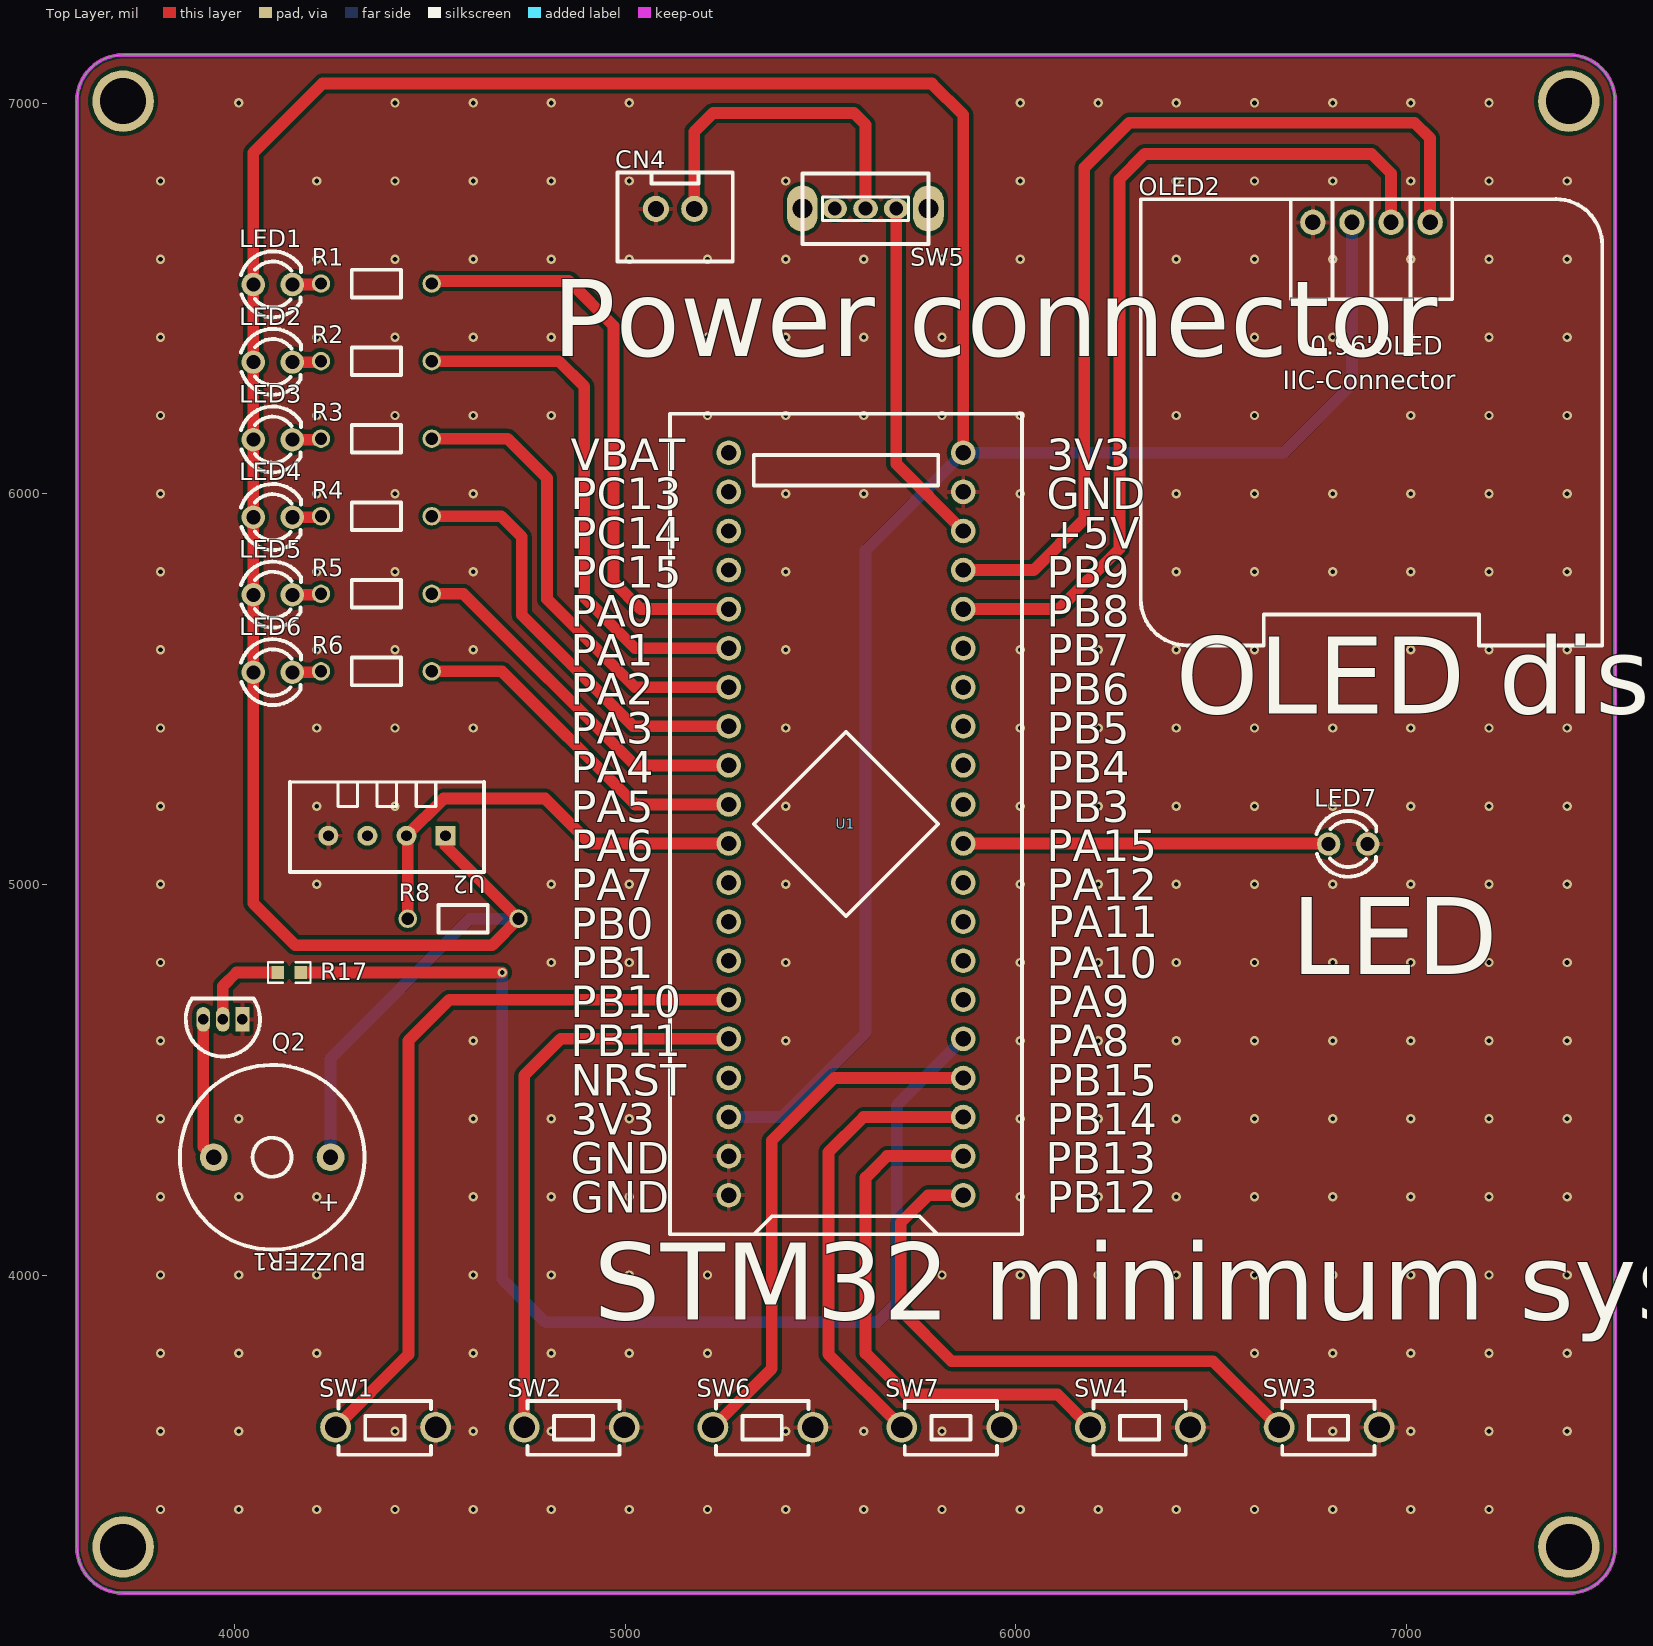
[diagram p0: Top Layer view]
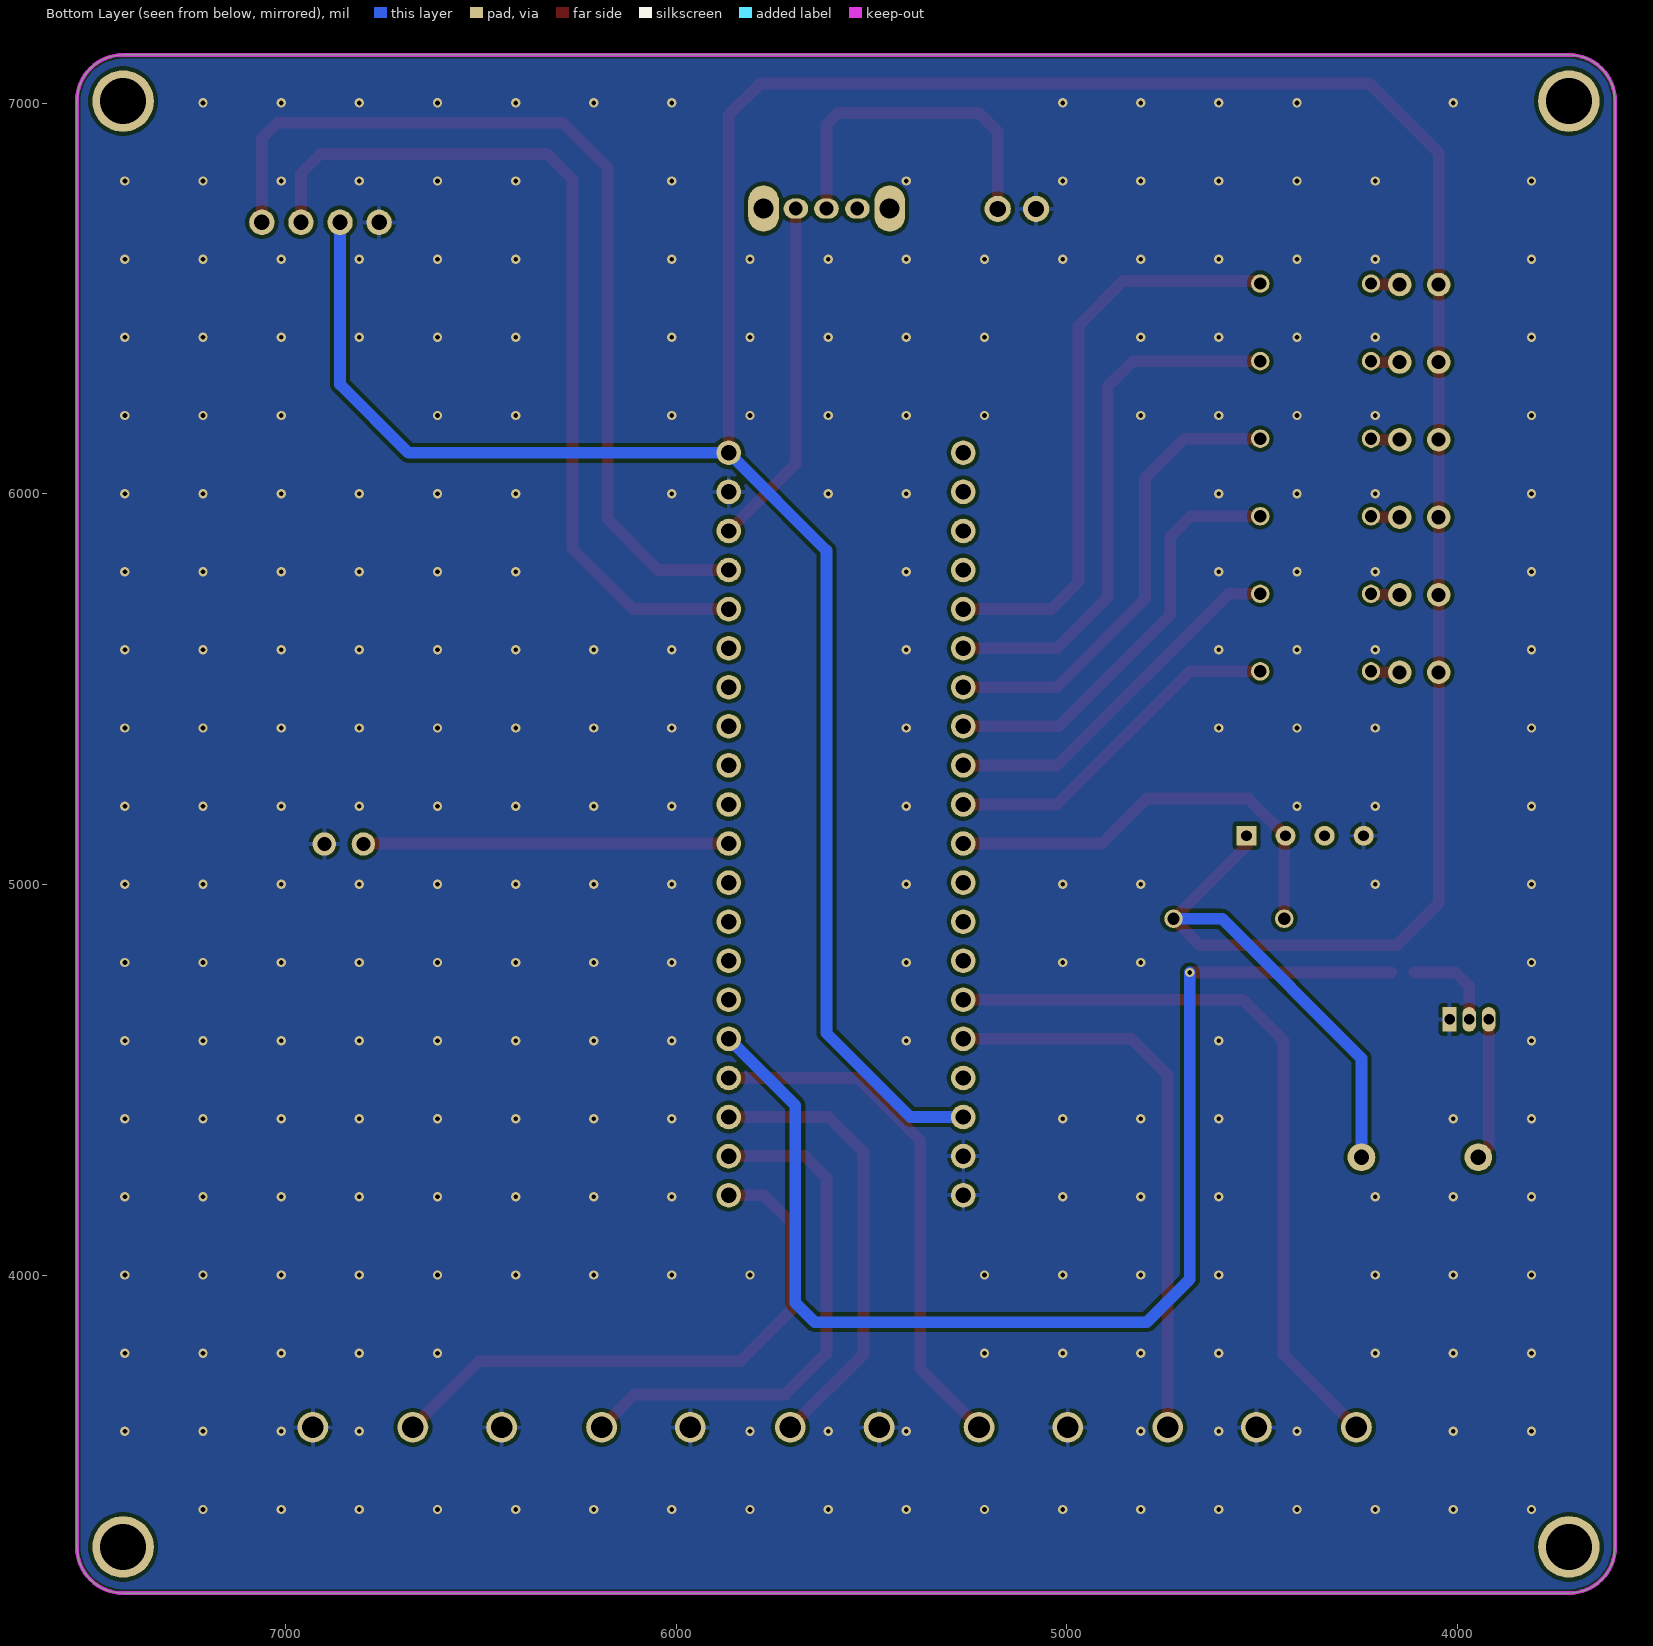
[diagram p1: Bottom Layer view, seen from below]
# Altium PCB MISC51258.pcbdoc
Units mil, origin at the board's own origin, x right, y up, seen from the top; angles counter-clockwise.
Board outline 3937.01 x 3937.01 mil, 2 copper layers (Top Layer, Bottom Layer), stack 62.206 mil thick; 28 components, 46 nets, 106 pads, 258 vias.

## Layer stack, top to bottom
Top Solder Mask Layer: solder mask 0.394, Dk 3.3
Top Layer: signal copper 1.379
Dielectric1: surface 59.449, FR4, Dk 4.5
Bottom Layer: signal copper 1.378
Bottom Solder Mask Layer: solder mask 0.394, Dk 3.3

## Board outline
3714.61,7123.5 ccw(c3714.61,7005.39) 3596.5,7005.39 3596.5,3304.61 ccw(c3714.61,3304.61) 3714.61,3186.5 7415.39,3186.5 ccw(c7415.39,3304.61) 7533.5,3304.61 7533.5,7005.39 ccw(c7415.39,7005.39) 7415.39,7123.5 3714.61,7123.5

## Design rules (kind name [scope] priority, off if disabled: settings)
BoardOutlineClearance copperThickness2oz_1 [All] p2 off: genericclearance=7.99 ignorepadtopadclearanceinfootprint=FALSE except(0: Arc-SplitContinuation Track-SplitContinuation SMDPad-SplitContinuation THPad-SplitContinuation Via-SplitContinuation Fill-SplitContinuation Region-SplitContinuation Poly-SplitContinuation Text-SplitContinuation Hole-SplitContinuation; 5.98: Arc-CutoutEdge Track-CutoutEdge SMDPad-CutoutEdge THPad-CutoutEdge Via-CutoutEdge Text-CutoutEdge; 6.9: Hole-OutlineEdge Hole-CutoutEdge; 10: Poly-OutlineEdge Poly-CutoutEdge; 11.81: Arc-OutlineEdge Track-OutlineEdge SMDPad-OutlineEdge THPad-OutlineEdge Via-OutlineEdge Fill-OutlineEdge Region-OutlineEdge Text-OutlineEdge Fill-CutoutEdge Region-CutoutEdge)
BoardOutlineClearance Plane_innerPlane_1 [All] p4 off: genericclearance=4.02 ignorepadtopadclearanceinfootprint=FALSE except(0: Arc-SplitContinuation Track-SplitContinuation SMDPad-SplitContinuation THPad-SplitContinuation Via-SplitContinuation Fill-SplitContinuation Region-SplitContinuation Poly-SplitContinuation Text-SplitContinuation Hole-SplitContinuation; 5.98: Arc-CutoutEdge Track-CutoutEdge SMDPad-CutoutEdge THPad-CutoutEdge Via-CutoutEdge Text-CutoutEdge; 6.9: Hole-OutlineEdge Hole-CutoutEdge; 10: Poly-OutlineEdge Poly-CutoutEdge; 11.81: Arc-OutlineEdge Track-OutlineEdge SMDPad-OutlineEdge THPad-OutlineEdge Via-OutlineEdge Fill-OutlineEdge Region-OutlineEdge Text-OutlineEdge Fill-CutoutEdge Region-CutoutEdge)
BoardOutlineClearance Copper_copperRegion_1 [All] p6 off: genericclearance=4.02 ignorepadtopadclearanceinfootprint=FALSE except(0: Arc-SplitContinuation Track-SplitContinuation SMDPad-SplitContinuation THPad-SplitContinuation Via-SplitContinuation Fill-SplitContinuation Region-SplitContinuation Poly-SplitContinuation Text-SplitContinuation Hole-SplitContinuation; 5.98: Arc-CutoutEdge Track-CutoutEdge SMDPad-CutoutEdge THPad-CutoutEdge Via-CutoutEdge Text-CutoutEdge; 6.9: Hole-OutlineEdge Hole-CutoutEdge; 10: Poly-OutlineEdge Poly-CutoutEdge; 11.81: Arc-OutlineEdge Track-OutlineEdge SMDPad-OutlineEdge THPad-OutlineEdge Via-OutlineEdge Fill-OutlineEdge Region-OutlineEdge Text-OutlineEdge Fill-CutoutEdge Region-CutoutEdge)
BoardOutlineClearance Copper_copperRegion_copperThickness1oz_1 [All] p8 off: genericclearance=4.02 ignorepadtopadclearanceinfootprint=FALSE except(0: Arc-SplitContinuation Track-SplitContinuation SMDPad-SplitContinuation THPad-SplitContinuation Via-SplitContinuation Fill-SplitContinuation Region-SplitContinuation Poly-SplitContinuation Text-SplitContinuation Hole-SplitContinuation; 5.98: Arc-CutoutEdge Track-CutoutEdge SMDPad-CutoutEdge THPad-CutoutEdge Via-CutoutEdge Text-CutoutEdge; 6.9: Hole-OutlineEdge Hole-CutoutEdge; 10: Poly-OutlineEdge Poly-CutoutEdge; 11.81: Arc-OutlineEdge Track-OutlineEdge SMDPad-OutlineEdge THPad-OutlineEdge Via-OutlineEdge Fill-OutlineEdge Region-OutlineEdge Text-OutlineEdge Fill-CutoutEdge Region-CutoutEdge)
BoardOutlineClearance Copper_copperRegion_Copper_copperRegion_1 [All] p10 off: genericclearance=4.02 ignorepadtopadclearanceinfootprint=FALSE except(0: Arc-SplitContinuation Track-SplitContinuation SMDPad-SplitContinuation THPad-SplitContinuation Via-SplitContinuation Fill-SplitContinuation Region-SplitContinuation Poly-SplitContinuation Text-SplitContinuation Hole-SplitContinuation; 5.98: Arc-CutoutEdge Track-CutoutEdge SMDPad-CutoutEdge THPad-CutoutEdge Via-CutoutEdge Text-CutoutEdge; 6.9: Hole-OutlineEdge Hole-CutoutEdge; 10: Poly-OutlineEdge Poly-CutoutEdge; 11.81: Arc-OutlineEdge Track-OutlineEdge SMDPad-OutlineEdge THPad-OutlineEdge Via-OutlineEdge Fill-OutlineEdge Region-OutlineEdge Text-OutlineEdge Fill-CutoutEdge Region-CutoutEdge)
BoardOutlineClearance copperThickness1oz_1 [All] p12: genericclearance=4.02 ignorepadtopadclearanceinfootprint=FALSE except(0: Arc-SplitContinuation Track-SplitContinuation SMDPad-SplitContinuation THPad-SplitContinuation Via-SplitContinuation Fill-SplitContinuation Region-SplitContinuation Poly-SplitContinuation Text-SplitContinuation Hole-SplitContinuation; 5.98: Arc-CutoutEdge Track-CutoutEdge SMDPad-CutoutEdge THPad-CutoutEdge Via-CutoutEdge Text-CutoutEdge; 6.9: Hole-OutlineEdge Hole-CutoutEdge; 10: Poly-OutlineEdge Poly-CutoutEdge; 11.81: Arc-OutlineEdge Track-OutlineEdge SMDPad-OutlineEdge THPad-OutlineEdge Via-OutlineEdge Fill-OutlineEdge Region-OutlineEdge Text-OutlineEdge Fill-CutoutEdge Region-CutoutEdge)
Clearance copperThickness2oz [All] p1 off: gap=7.99 ignorepadtopadclearanceinfootprint=FALSE except(5.98: SMDPad-Track SMDPad-SMDPad THPad-Track SMDPad-THPad THPad-THPad Track-Via SMDPad-Via THPad-Via Via-Via Fill-SMDPad Region-SMDPad Fill-THPad Region-THPad Fill-Via Region-Via Fill-Fill Fill-Region Region-Region Arc-Track Arc-SMDPad Arc-THPad Arc-Via Fill-Arc Region-Arc Arc-Arc Text-Track SMDPad-Text Text-THPad Text-Via Fill-Text Region-Text Arc-Text Text-Text; 6.9: Hole-Track Hole-SMDPad Hole-THPad Hole-Via Fill-Hole Region-Hole Hole-Arc Hole-Text; 10: Poly-Track Poly-SMDPad Poly-THPad Poly-Via Poly-Fill Poly-Region Poly-Poly Poly-Arc Poly-Text Poly-Hole; 11.81: Fill-Track Region-Track)
Clearance Plane_innerPlane [All] p3 off: gap=4.02 ignorepadtopadclearanceinfootprint=FALSE except(5.98: SMDPad-Track SMDPad-SMDPad THPad-Track SMDPad-THPad THPad-THPad Track-Via SMDPad-Via THPad-Via Via-Via Fill-SMDPad Region-SMDPad Fill-THPad Region-THPad Fill-Via Region-Via Fill-Fill Fill-Region Region-Region Arc-Track Arc-SMDPad Arc-THPad Arc-Via Fill-Arc Region-Arc Arc-Arc Text-Track SMDPad-Text Text-THPad Text-Via Fill-Text Region-Text Arc-Text Text-Text; 6.9: Hole-Track Hole-SMDPad Hole-THPad Hole-Via Fill-Hole Region-Hole Hole-Arc Hole-Text; 10: Poly-Track Poly-SMDPad Poly-THPad Poly-Via Poly-Fill Poly-Region Poly-Poly Poly-Arc Poly-Text Poly-Hole; 11.81: Fill-Track Region-Track)
Clearance Copper_copperRegion [All] p5 off: gap=4.02 ignorepadtopadclearanceinfootprint=FALSE except(5.98: SMDPad-Track SMDPad-SMDPad THPad-Track SMDPad-THPad THPad-THPad Track-Via SMDPad-Via THPad-Via Via-Via Fill-SMDPad Region-SMDPad Fill-THPad Region-THPad Fill-Via Region-Via Fill-Fill Fill-Region Region-Region Arc-Track Arc-SMDPad Arc-THPad Arc-Via Fill-Arc Region-Arc Arc-Arc Text-Track SMDPad-Text Text-THPad Text-Via Fill-Text Region-Text Arc-Text Text-Text; 6.9: Hole-Track Hole-SMDPad Hole-THPad Hole-Via Fill-Hole Region-Hole Hole-Arc Hole-Text; 10: Poly-Track Poly-SMDPad Poly-THPad Poly-Via Poly-Fill Poly-Region Poly-Poly Poly-Arc Poly-Text Poly-Hole; 11.81: Fill-Track Region-Track)
Clearance Copper_copperRegion_copperThickness1oz [All] p7 off: gap=4.02 ignorepadtopadclearanceinfootprint=FALSE except(5.98: SMDPad-Track SMDPad-SMDPad THPad-Track SMDPad-THPad THPad-THPad Track-Via SMDPad-Via THPad-Via Via-Via Fill-SMDPad Region-SMDPad Fill-THPad Region-THPad Fill-Via Region-Via Fill-Fill Fill-Region Region-Region Arc-Track Arc-SMDPad Arc-THPad Arc-Via Fill-Arc Region-Arc Arc-Arc Text-Track SMDPad-Text Text-THPad Text-Via Fill-Text Region-Text Arc-Text Text-Text; 6.9: Hole-Track Hole-SMDPad Hole-THPad Hole-Via Fill-Hole Region-Hole Hole-Arc Hole-Text; 10: Poly-Track Poly-SMDPad Poly-THPad Poly-Via Poly-Fill Poly-Region Poly-Poly Poly-Arc Poly-Text Poly-Hole; 11.81: Fill-Track Region-Track)
Clearance Copper_copperRegion_Copper_copperRegion [All] p9 off: gap=4.02 ignorepadtopadclearanceinfootprint=FALSE except(5.98: SMDPad-Track SMDPad-SMDPad THPad-Track SMDPad-THPad THPad-THPad Track-Via SMDPad-Via THPad-Via Via-Via Fill-SMDPad Region-SMDPad Fill-THPad Region-THPad Fill-Via Region-Via Fill-Fill Fill-Region Region-Region Arc-Track Arc-SMDPad Arc-THPad Arc-Via Fill-Arc Region-Arc Arc-Arc Text-Track SMDPad-Text Text-THPad Text-Via Fill-Text Region-Text Arc-Text Text-Text; 6.9: Hole-Track Hole-SMDPad Hole-THPad Hole-Via Fill-Hole Region-Hole Hole-Arc Hole-Text; 10: Poly-Track Poly-SMDPad Poly-THPad Poly-Via Poly-Fill Poly-Region Poly-Poly Poly-Arc Poly-Text Poly-Hole; 11.81: Fill-Track Region-Track)
Clearance copperThickness1oz [All] p11: gap=4.02 ignorepadtopadclearanceinfootprint=FALSE except(5.98: SMDPad-Track SMDPad-SMDPad THPad-Track SMDPad-THPad THPad-THPad Track-Via SMDPad-Via THPad-Via Via-Via Fill-SMDPad Region-SMDPad Fill-THPad Region-THPad Fill-Via Region-Via Fill-Fill Fill-Region Region-Region Arc-Track Arc-SMDPad Arc-THPad Arc-Via Fill-Arc Region-Arc Arc-Arc Text-Track SMDPad-Text Text-THPad Text-Via Fill-Text Region-Text Arc-Text Text-Text; 6.9: Hole-Track Hole-SMDPad Hole-THPad Hole-Via Fill-Hole Region-Hole Hole-Arc Hole-Text; 10: Poly-Track Poly-SMDPad Poly-THPad Poly-Via Poly-Fill Poly-Region Poly-Poly Poly-Arc Poly-Text Poly-Hole; 11.81: Fill-Track Region-Track)
DiffPairsRouting differentialPair [All] p1: maxlimit=6 minlimit=6 mostfreqgap=6 toplayer_minwidth=5 toplayer_prefwidth=10 toplayer_maxwidth=100 toplayer_mingap=6 toplayer_prefgap=6 toplayer_maxgap=6 bottomlayer_minwidth=5 bottomlayer_prefwidth=10 bottomlayer_maxwidth=100 bottomlayer_mingap=6 bottomlayer_prefgap=6 bottomlayer_maxgap=6 maxuncoupledlength=10
HoleToHoleClearance otherClearance [All] p1: gap=11.81 allowstackedmicrovias=TRUE
Length netLength [All] p1: minlimit=0 maxlimit=0
PasteMaskExpansion pasteMaskExpansion [All] p1: expansion=0
PlaneConnect innerPlane [All] p1: planeconnectstyle=Relief reliefexpansion=20 reliefentries=4 reliefconductorwidth=10 reliefairgap=10
PolygonConnect copperRegion_copperThickness1oz [All] p1 off: connectstyle=Relief reliefconductorwidth=10 reliefentries=4 polygonreliefangle="90 Angle" airgapwidth=10 via.connectstyle=Relief via.reliefconductorwidth=10 via.reliefentries=4 via.polygonreliefangle="90 Angle" via.airgapwidth=10
PolygonConnect copperRegion_Copper_copperRegion [All] p2 off: connectstyle=Relief reliefconductorwidth=10 reliefentries=4 polygonreliefangle="90 Angle" airgapwidth=10 via.connectstyle=Relief via.reliefconductorwidth=10 via.reliefentries=4 via.polygonreliefangle="90 Angle" via.airgapwidth=10
PolygonConnect copperRegion [All] p3: connectstyle=Relief reliefconductorwidth=10 reliefentries=4 polygonreliefangle="90 Angle" airgapwidth=10 via.connectstyle=Relief via.reliefconductorwidth=10 via.reliefentries=4 via.polygonreliefangle="90 Angle" via.airgapwidth=10
RoutingVias viaSize [All] p1: holewidth=12.01 width=24.02 viastyle="Through Hole" minholewidth=11.81 minwidth=19.68 maxholewidth=248.03 maxwidth=393.7
SolderMaskExpansion solderMaskExpansion [IsVia] p1: expansion=-1000 istentingtop=TRUE
SolderMaskExpansion solderMaskExpansion [All] p2: expansion=2 istentingtop=FALSE
Width copperThickness2oz_2 [All] p1 off: maxlimit=100 minlimit=8 preferedwidth=10
Width copperThickness1oz_2 [All] p2: maxlimit=100 minlimit=5 preferedwidth=10

## Components (designator, comment, footprint, x,y, rotation, side; value= is the part's Value field where it differs from the comment)
BUZZER1 "2.4kHz" BUZ-TH_BD12.0-P7.60-D0.6-FD 4096.11,4302.06 r180 top
CN4 "XH2.54*2P_through-hole" CONN-TH_2P-P2.50-XH2.54-2P 5127.54,6729.39 r0 top
LED1 "" LED_TH-3mm 4097.99,6535.66 r0 top
LED2 "" LED_TH-3mm 4097.99,6337.16 r0 top
LED3 "" LED_TH-3mm 4097.99,6138.66 r0 top
LED4 "" LED_TH-3mm 4097.99,5940.16 r0 top
LED5 "" LED_TH-3mm 4097.99,5741.66 r0 top
LED6 "" LED_TH-3mm 4097.99,5543.16 r0 top
LED7 "" LED_TH-3mm 6850.19,5103.75 r0 top
OLED2 "" 0.96OLED_4P 6910,6695 r0 top
Q2 "" S8050_TO_92 3970,4655 r180 top
R1 "220Ω" Res_1/8W 4362.97,6535.66 r0 top
R2 "220Ω" Res_1/8W 4362.97,6337.16 r0 top
R3 "220Ω" Res_1/8W 4362.97,6138.66 r0 top
R4 "220Ω" Res_1/8W 4362.97,5940.16 r0 top
R5 "220Ω" Res_1/8W 4362.97,5741.66 r0 top
R6 "220Ω" Res_1/8W 4362.97,5543.16 r0 top
R8 "4.7kΩ" Res_1/8W 4585,4910 r0 top
R17 "1kΩ" R0603 4140,4775 r180 top
SW1 "" Key_TH_3.5x6x4.3 4380,3610.71 r0 top
SW2 "" Key_TH_3.5x6x4.3 4863,3610.71 r0 top
SW3 "" Key_TH_3.5x6x4.3 6795,3610.71 r0 top
SW4 "" Key_TH_3.5x6x4.3 6312,3610.71 r0 top
SW5 "" 拨动开关 5620,6730 r180 top
SW6 "" Key_TH_3.5x6x4.3 5346,3610.71 r0 top
SW7 "" Key_TH_3.5x6x4.3 5829,3610.71 r0 top
U1 "STM32F103C8T6-Card" CONN-TH_L53.3-W22.9_STM32F103C8T6-CARD 5565,5155 r90 top
U2 "DHT11" SENSOR-TH_DHT11 4390,5125 r180 top

## Footprints (in the part's own frame and the unit in brackets; to place one, negate y for a bottom-side part, rotate by r counter-clockwise, add the part's x,y. Pads: shape width x height; smd on the part's side, far side on the other; paste and mask are expansions set on the pad)
0.96OLED_4P [mm]
  round 1.65 hole 1 copper offset 0,0: 1(-3.81,-0.001) 2(-1.27,0.002) 3(1.27,0.002) 4(3.81,0.002)
  silkscreen extent -15,-27.5 15,1.5
BUZ-TH_BD12.0-P7.60-D0.6-FD [mm]
  round 1.8 hole 1: 1(-3.8,0) 2(3.8,0)
  silkscreen extent -6,-6 6,6
CONN-TH_2P-P2.50-XH2.54-2P [mm]
  round 1.7 hole 1.05 paste+0 mask+0.05: 1(1.25,0) 2(-1.25,0)
  silkscreen extent -3.75,-3.42 3.75,2.37
CONN-TH_L53.3-W22.9_STM32F103C8T6-CARD [mm]
  round 1.6 hole 1: 1(-24.13,-7.62) 2(-21.59,-7.62) 3(-19.05,-7.62) 4(-16.51,-7.62) 5(-13.97,-7.62) 6(-11.43,-7.62) 7(-8.89,-7.62) 8(-6.35,-7.62) 9(-3.81,-7.62) 10(-1.27,-7.62) 11(1.27,-7.62) 12(3.81,-7.62) 13(6.35,-7.62) 14(8.89,-7.62) 15(11.43,-7.62) 16(13.97,-7.62) 17(16.51,-7.62) 18(19.05,-7.62) 19(21.59,-7.62) 20(24.13,-7.62) 21(24.13,7.62) 22(21.59,7.62) 23(19.05,7.62) 24(16.51,7.62) 25(13.97,7.62) 26(11.43,7.62) 27(8.89,7.62) 28(6.35,7.62) 29(3.81,7.62) 30(1.27,7.62) 31(-1.27,7.62) 32(-3.81,7.62) 33(-6.35,7.62) 34(-8.89,7.62) 35(-11.43,7.62) 36(-13.97,7.62) 37(-16.51,7.62) 38(-19.05,7.62) 39(-21.59,7.62) 40(-24.13,7.62)
  silkscreen extent -26.67,-11.43 26.67,11.43
Key_TH_3.5x6x4.3 [mil]
  round 78.7 hole 55.1 paste+0 mask+2: A(-121.44,0) B(134.46,0)
  silkscreen extent -114,-70 123,68
LED_TH-3mm [mil]
  round 60 hole 36 paste+0 mask+2: 1(-50,0) 2(50,0)
  silkscreen extent -81,-84 72,85
R0603 [mil]
  rect 31.75x34.02 smd paste-3937.01 mask+2: 1(-29.66,0) 2(29.66,0)
  silkscreen extent -55,-26 55,26
Res_1/8W [mil]
  round 47.2 hole 31.5 paste+0 mask+2: 1(-141.7,2.48) 2(141.7,2.48)
  silkscreen extent -63,-33 63,38
S8050_TO_92 [mil]
  rect 35.4x63 hole 27.6 paste+0 mask+2: 1(-50,0)
  oval 35.4x63 hole 27.6 paste+0 mask+2: 2(0,0) 3(50,0)
  silkscreen extent -95,-53 95,95
SENSOR-TH_DHT11 [mil]
  rect 51x51 hole 28: 1(-150,0)
  round 51 hole 28: 2(-50,0) 3(50,0) 4(150,0)
  silkscreen extent -248,-138 248,93
拨动开关 [mil]
  oval 63x51.2 hole 35.4 paste+0 mask+2: 1(-73.4,0) 2(5,0) 3(84,0)
  oval 78.7x118.1 hole 51.2 paste+0 mask+2: 4(166.7,0) 5(-156.1,0)
  silkscreen extent -156,-90 167,90

## Free pads (board coordinates)
  round 157.48 hole 118.11: 1(3714.61,7005.39) 1(3714.61,3304.61) 1(7415.39,7005.39) 1(7415.39,3304.61)

## Via types
v1: diameter 24.02, hole 12, Top Layer to Bottom Layer, 258 vias

## Nets (pads, with @x,y where several pads share a name; then routed paths per layer and width w, separated by ;. In a path a pad name is that pad's centre, name@x,y a point inside that pad or via, vN(x,y) a via of type N, cw(c..) or ccw(c..) an arc to the next point about the centre after c; other vN are vias at no path point)
$1N17118: CN4.1 SW5.2 | length 883
  Top Layer w30: CN4.1 5176.76,6926.76 5225,6975 5585,6975 5615,6945 SW5.2
$1N17244: LED1.2 R1.1 | length 74.3
  Top Layer w30: LED1.2 4218.8,6535.66 R1.1
$1N17247: LED2.2 R2.1 | length 74.3
  Top Layer w30: LED2.2 4218.8,6337.16 R2.1
$1N17250: LED3.2 R3.1 | length 74.3
  Top Layer w30: LED3.2 4218.8,6138.66 R3.1
$1N17253: LED4.2 R4.1 | length 74.3
  Top Layer w30: LED4.2 4218.8,5940.16 R4.1
$1N17256: LED5.2 R5.1 | length 74.3
  Top Layer w30: LED5.2 4218.8,5741.66 R5.1
$1N17259: LED6.2 R6.1 | length 74.3
  Top Layer w30: LED6.2 4218.8,5543.16 R6.1
$1N17277: Q2.2 R17.2 | length 239.8
  Top Layer w30: Q2.2 3970,4740 4005,4775 R17.2
$1N17287: BUZZER1.2 Q2.3 | length 363.9
  Top Layer w30: Q2.3 3920,4328.57 BUZZER1.2
+5V: SW5.1 U1.18 | length 896.1
  Top Layer w30: SW5.1 5693.4,6076.6 U1.18
GND: CN4.2 LED7.2 OLED2.1 Q2.1 SW1.B SW2.B SW3.B SW4.B SW6.B SW7.B U1.19 U1.39 U1.40 U2.4
  other v1: 3810.6,3400.6 4010.6,3400.6 4210.6,3400.6 4410.6,3400.6 4610.6,3400.6 4810.6,3400.6 5010.6,3400.6 5210.6,3400.6 5410.6,3400.6 5610.6,3400.6 5810.6,3400.6 6010.6,3400.6 6210.6,3400.6 6410.6,3400.6 6610.6,3400.6 6810.6,3400.6 7010.6,3400.6 7210.6,3400.6 3810.6,3600.6 4010.6,3600.6 4410.6,3600.6 4610.6,3600.6 4810.6,3600.6 5410.6,3600.6 5610.6,3600.6 5810.6,3600.6 6810.6,3600.6 7010.6,3600.6 7210.6,3600.6 7410.6,3600.6 3810.6,3800.6 4010.6,3800.6 4210.6,3800.6 4610.6,3800.6 4810.6,3800.6 5010.6,3800.6 5210.6,3800.6 6610.6,3800.6 6810.6,3800.6 7010.6,3800.6 7210.6,3800.6 7410.6,3800.6 3810.6,4000.6 4010.6,4000.6 4210.6,4000.6 4610.6,4000.6 4810.6,4000.6 5010.6,4000.6 5210.6,4000.6 5810.6,4000.6 6010.6,4000.6 6210.6,4000.6 6410.6,4000.6 6610.6,4000.6 6810.6,4000.6 7010.6,4000.6 7210.6,4000.6 7410.6,4000.6 3810.6,4200.6 4010.6,4200.6 4210.6,4200.6 4610.6,4200.6 4810.6,4200.6 5010.6,4200.6 6010.6,4200.6 6210.6,4200.6 6410.6,4200.6 6610.6,4200.6 6810.6,4200.6 7010.6,4200.6 7210.6,4200.6 7410.6,4200.6 3810.6,4400.6 4010.6,4400.6 4610.6,4400.6 4810.6,4400.6 5010.6,4400.6 6010.6,4400.6 6210.6,4400.6 6410.6,4400.6 6610.6,4400.6 6810.6,4400.6 7010.6,4400.6 7210.6,4400.6 7410.6,4400.6 3810.6,4600.6 4610.6,4600.6 5410.6,4600.6 6010.6,4600.6 6210.6,4600.6 6410.6,4600.6 6610.6,4600.6 6810.6,4600.6 7010.6,4600.6 7210.6,4600.6 7410.6,4600.6 3810.6,4800.6 4810.6,4800.6 5010.6,4800.6 5410.6,4800.6 6010.6,4800.6 6210.6,4800.6 6410.6,4800.6 6610.6,4800.6 6810.6,4800.6 7010.6,4800.6 7210.6,4800.6 7410.6,4800.6 3810.6,5000.6 4210.6,5000.6 4810.6,5000.6 5010.6,5000.6 5410.6,5000.6 6010.6,5000.6 6210.6,5000.6 6410.6,5000.6 6610.6,5000.6 6810.6,5000.6 7010.6,5000.6 7210.6,5000.6 7410.6,5000.6 3810.6,5200.6 4210.6,5200.6 4410.6,5200.6 5410.6,5200.6 6010.6,5200.6 6210.6,5200.6 6410.6,5200.6 6610.6,5200.6 6810.6,5200.6 7010.6,5200.6 7210.6,5200.6 7410.6,5200.6 3810.6,5400.6 4210.6,5400.6 4410.6,5400.6 4610.6,5400.6 5410.6,5400.6 6010.6,5400.6 6210.6,5400.6 6410.6,5400.6 6610.6,5400.6 6810.6,5400.6 7010.6,5400.6 7210.6,5400.6 7410.6,5400.6 3810.6,5600.6 4210.6,5600.6 4410.6,5600.6 4610.6,5600.6 5410.6,5600.6 6010.6,5600.6 6210.6,5600.6 6410.6,5600.6 6610.6,5600.6 6810.6,5600.6 7010.6,5600.6 7210.6,5600.6 7410.6,5600.6 3810.6,5800.6 4210.6,5800.6 4410.6,5800.6 4610.6,5800.6 5410.6,5800.6 6410.6,5800.6 6610.6,5800.6 6810.6,5800.6 7010.6,5800.6 7210.6,5800.6 7410.6,5800.6 3810.6,6000.6 4210.6,6000.6 4410.6,6000.6 4610.6,6000.6 5410.6,6000.6 5610.6,6000.6 6010.6,6000.6 6410.6,6000.6 6610.6,6000.6 6810.6,6000.6 7010.6,6000.6 7210.6,6000.6 7410.6,6000.6 3810.6,6200.6 4210.6,6200.6 4410.6,6200.6 4610.6,6200.6 4810.6,6200.6 5210.6,6200.6 5410.6,6200.6 5610.6,6200.6 5810.6,6200.6 6010.6,6200.6 6410.6,6200.6 6610.6,6200.6 7010.6,6200.6 7210.6,6200.6 7410.6,6200.6 3810.6,6400.6 4210.6,6400.6 4410.6,6400.6 4610.6,6400.6 4810.6,6400.6 5210.6,6400.6 5410.6,6400.6 5610.6,6400.6 5810.6,6400.6 6010.6,6400.6 6410.6,6400.6 6610.6,6400.6 6810.6,6400.6 7010.6,6400.6 7210.6,6400.6 7410.6,6400.6 3810.6,6600.6 4210.6,6600.6 4410.6,6600.6 4610.6,6600.6 4810.6,6600.6 5010.6,6600.6 5210.6,6600.6 5410.6,6600.6 5610.6,6600.6 5810.6,6600.6 6010.6,6600.6 6410.6,6600.6 6610.6,6600.6 6810.6,6600.6 7010.6,6600.6 7210.6,6600.6 7410.6,6600.6 3810.6,6800.6 4210.6,6800.6 4410.6,6800.6 4610.6,6800.6 4810.6,6800.6 5010.6,6800.6 5410.6,6800.6 6010.6,6800.6 6410.6,6800.6 6610.6,6800.6 6810.6,6800.6 7010.6,6800.6 7210.6,6800.6 7410.6,6800.6 4010.6,7000.6 4410.6,7000.6 4610.6,7000.6 4810.6,7000.6 5010.6,7000.6 6010.6,7000.6 6210.6,7000.6 6410.6,7000.6 6610.6,7000.6 6810.6,7000.6 7010.6,7000.6 7210.6,7000.6
NRST: U1.37
PA0: R1.2 U1.25 | length 1494.8
  Top Layer w30: R1.2 4511.54,6545 4855,6545 4970,6430 4970,5775 5040,5705 U1.25
PA1: R2.2 U1.26 | length 1380.9
  Top Layer w30: R2.2 4830.36,6339.64 4895,6275 4895,5735 5025,5605 U1.26
PA2: R3.2 U1.27 | length 1205.4
  Top Layer w30: R3.2 4698.87,6141.13 4800,6040 4800,5730 5025,5505 U1.27
PA3: R4.2 U1.28 | length 1100.2
  Top Layer w30: R4.2 4682.37,5942.63 4735,5890 4735,5690 5020,5405 U1.28
PA4: R5.2 U1.29 | length 942.2
  Top Layer w30: R5.2 4585.87,5744.13 5025,5305 U1.29
PA5: R6.2 U1.30 | length 901.4
  Top Layer w30: R6.2 4684.37,5545.63 5025,5205 U1.30
PA6: R8.1 U1.31 U2.2 | length 1125.9
  Top Layer w30: R8.1 4443.3,5121.7 U2.2 4535,5220 4795,5220 4910,5105 U1.31
PA7: U1.32
PA8: R17.1 U1.5 | length 3122
  Top Layer w30: R17.1 v1(4685,4775)
  Bottom Layer w30: v1(4685,4775) 4685,3990 4795,3880 5645,3880 5695,3930 5695,4435 U1.5
PA9: U1.6
PA10: U1.7
PA11: U1.8
PA12: U1.9
PA15: LED7.1 U1.10 | length 935.7
  Top Layer w30: U1.10 6798.93,5105 LED7.1
PB0: U1.33
PB1: U1.34
PB3: U1.11
PB4: U1.12
PB5: U1.13
PB6: U1.14
PB7: U1.15
PB8: OLED2.3 U1.16 | length 2276.8
  Top Layer w30: U1.16 6110,5705 6265,5860 6265,6805 6330,6870 6910,6870 6960,6820 OLED2.3@6960,6695.05
PB9: OLED2.4 U1.17 | length 2428
  Top Layer w30: U1.17 6045,5805 6175,5935 6175,6835 6290,6950 7020,6950 7060,6910 OLED2.4@7060,6695.05
PB10: SW1.A U1.35 | length 1930
  Top Layer w30: SW1.A 4445,3797.15 4445,4600 4550,4705 U1.35
PB11: SW2.A U1.36 | length 1463
  Top Layer w30: SW2.A 4741.56,4511.56 4835,4605 U1.36
PB12: SW3.A U1.1 | length 1506.5
  Top Layer w30: U1.1 5775,4205 5705,4135 5705,3910 5835,3780 6504.27,3780 SW3.A
PB13: SW4.A U1.2 | length 1376.7
  Top Layer w30: U1.2 5670,4305 5615,4250 5615,3800 5720,3695 6106.27,3695 SW4.A
PB14: SW7.A U1.3 | length 1164.3
  Top Layer w30: SW7.A 5520,3798.27 5520,4315 5610,4405 U1.3
PB15: SW6.A U1.4 | length 1352.9
  Top Layer w30: SW6.A 5375,3761.15 5375,4345 5535,4505 U1.4
PC13: U1.22
PC14: U1.23
PC15: U1.24
VBAT: U1.21
VCC: BUZZER1.1 LED1.1 LED2.1 LED3.1 LED4.1 LED5.1 LED6.1 OLED2.2 R8.2 U1.20 U1.38 U2.1 | length 10142.6
  Top Layer w30: U2.1 4540,5099.18 R8.2 4659.22,4845 4155.41,4845 4047.99,4952.42 LED6.1 LED5.1 LED4.1 LED3.1 LED2.1 LED1.1 4047.99,6872.99 4225,7050 5785,7050 5865,6970 U1.20
  Bottom Layer w30: BUZZER1.1 4245.72,4555.72 4602.48,4912.48 R8.2 ; U1.38 5400,4405 5615,4620 5615,5855 U1.20 6685,6105 6860,6280 OLED2.2@6860,6695.05
pads on no net: SW5.3 SW5.4 SW5.5 U2.3

## Polygon pours and split planes (outlines as drawn)
GND on Bottom Layer (solid, remove dead copper, pour order 2): 3525,7245 3525,3080 7700,3080 7700,7245
GND on Top Layer (solid, remove dead copper, pour order 2): 3000,7415 3000,3000 7930,3000 7930,7415

## Keep-outs
Board Outline Layer:
  the board outline again, w10

## Silkscreen, mask and mechanical layers (free items; w line width, h text height)
Top Silkscreen Layer:
  text "Power connector" at 4812.87,6351.57 h196.85
  text "VBAT" at 4860.95,6060 h80
  text "3V3" at 6079.16,6060 h80
  text "PC13" at 4860.95,5960 h80
  text "GND" at 6079.16,5960 h80
  text "PC14" at 4860.95,5860 h80
  text "+5V" at 6079.16,5860 h80
  text "PC15" at 4860.95,5760 h80
  text "PB9" at 6079.16,5760 h80
  text "PA0" at 4860.95,5660 h80
  text "PB8" at 6079.16,5660 h80
  text "PA1" at 4860.95,5560 h80
  text "PB7" at 6079.16,5560 h80
  text "PA2" at 4860.95,5460 h80
  text "PB6" at 6079.16,5460 h80
  text "OLED display" at 6408.66,5436.57 h196.85
  text "PA3" at 4860.95,5360 h80
  text "PB5" at 6079.16,5360 h80
  text "PA4" at 4860.95,5260 h80
  text "PB4" at 6079.16,5260 h80
  text "PA5" at 4860.95,5160 h80
  text "PB3" at 6079.16,5160 h80
  text "PA6" at 4860.95,5060 h80
  text "PA15" at 6079.16,5060 h80
  text "PA7" at 4860.95,4960 h80
  text "PA12" at 6079.16,4960 h80
  text "PA11" at 6080.95,4865 h80
  text "PB0" at 4860.95,4860 h80
  text "LED" at 6705,4770 h196.85
  text "PB1" at 4860.95,4760 h80
  text "PA10" at 6079.16,4760 h80
  text "PB10" at 4860.95,4660 h80
  text "PA9" at 6079.16,4660 h80
  text "PB11" at 4860.95,4560 h80
  text "PA8" at 6079.16,4560 h80
  text "NRST" at 4860.95,4460 h80
  text "PB15" at 6079.16,4460 h80
  text "3V3" at 4860.95,4360 h80
  text "PB14" at 6079.16,4360 h80
  text "GND" at 4860.95,4260 h80
  text "PB13" at 6075.95,4260 h80
  text "GND" at 4860.95,4160 h80
  text "PB12" at 6079.16,4160 h80
  text "STM32 minimum system" at 4919.45,3886.57 h196.85